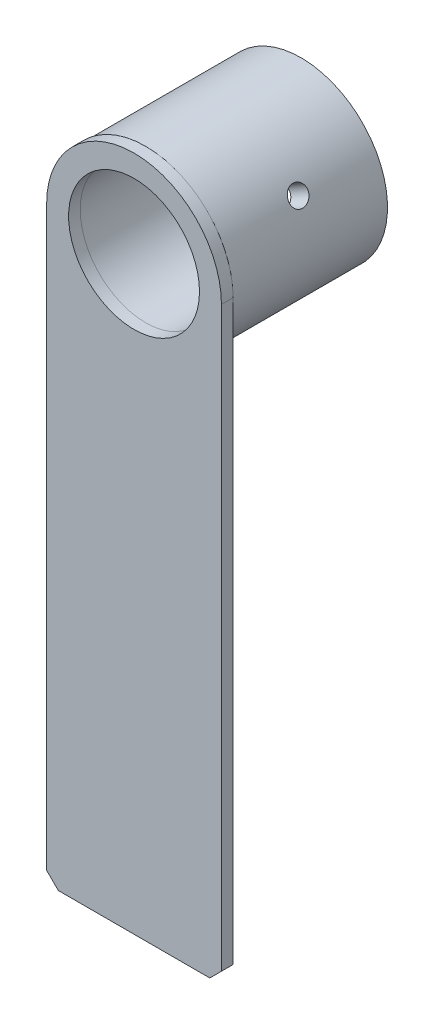
from build123d import *

# Parameters (mm, degrees)
EXTRUDE_1_DEPTH = 3
SKETCH_2_R      = 22.25
EXTRUDE_2_DEPTH = 40
SKETCH_3_W      = 16.85
SKETCH_3_H      = 43
SKETCH_5_W      = 2.5
SKETCH_5_H      = 22.5
SKETCH_6_W      = 2.5
SKETCH_6_H      = 14.072063551
CHAMFER_1_SIZE  = 3


with BuildPart() as part:
    # 草图1 → 凸台-拉伸1 (new body)
    with BuildSketch(Plane(origin=(0, 0, 20), x_dir=(-1, 0, 0), z_dir=(0, 0, -1))):
        with BuildLine():
            Line((-22.5, 0), (-22.5, -151.685393258))
            Line((-22.5, -151.685393258), (22.5, -151.685393258))
            Line((22.5, -151.685393258), (22.5, 0))
            ThreePointArc((22.5, 0), (0, 22.5), (-22.5, 0))
        make_face()
    extrude(amount=-EXTRUDE_1_DEPTH)


with BuildPart() as body_2:
    # 草图2 → 凸台-拉伸2 (new body)
    with BuildSketch(Plane(origin=(0, 0, 20), x_dir=(-1, 0, 0), z_dir=(0, 0, -1))):
        Circle(SKETCH_2_R)
    extrude(amount=EXTRUDE_2_DEPTH)


with BuildPart() as hole_wizard_m30_1_tool:
    # 草图3 → M30 间隙孔1 (revolve)
    with BuildSketch(Plane(origin=(0, 0, 23), x_dir=(0, -1, 0), z_dir=(1, 0, 0))):
        with Locations((8.425, 21.5)):
            Rectangle(SKETCH_3_W, SKETCH_3_H)
    revolve(axis=Axis((0, 0, 29.35), (0, 0, -1)))


with BuildPart() as part_1:
    add(part.part)

    # M30 间隙孔1: cut by hole_wizard_m30_1_tool
    add(hole_wizard_m30_1_tool.part, mode=Mode.SUBTRACT)

    # 倒角1
    chamfer_1_edges = [part_1.edges().sort_by_distance(p)[0] for p in [
        (-22.5, -151.685393258, 21.5),
        (22.5, -151.685393258, 21.5),
    ]]
    chamfer(chamfer_1_edges, length=CHAMFER_1_SIZE)


with BuildPart() as body_2_1:
    add(body_2.part)

    # M30 间隙孔1: cut by hole_wizard_m30_1_tool
    add(hole_wizard_m30_1_tool.part, mode=Mode.SUBTRACT)

    # 草图5 → Ø5.0 (5) 直径孔1 (revolve, cut)
    with BuildSketch(Plane(origin=(-19.485571585, 11.25, 0), x_dir=(-0.4999999999999359, -0.8660254037844758, 0), z_dir=(0, 0, 1))):
        with Locations((1.25, 11.25)):
            Rectangle(SKETCH_5_W, SKETCH_5_H)
    revolve(axis=Axis((-24.984832899, 14.425, 0), (0.8660254037844757, -0.4999999999999359, 0)), mode=Mode.SUBTRACT)

    # 草图6 → Ø5.0 (5) 直径孔2 (revolve, cut)
    with BuildSketch(Plane(origin=(14.431021274, 8.331754017, 0), x_dir=(0.5000000000000044, -0.8660254037844362, 0), z_dir=(0, 0, 1))):
        with Locations((1.25, 7.036031776)):
            Rectangle(SKETCH_6_W, SKETCH_6_H)
    revolve(axis=Axis((8.93175996, 5.156754017, 0), (0.866025403784436, 0.5000000000000044, 0)), mode=Mode.SUBTRACT)


solid = Compound([part_1.part, body_2_1.part])
